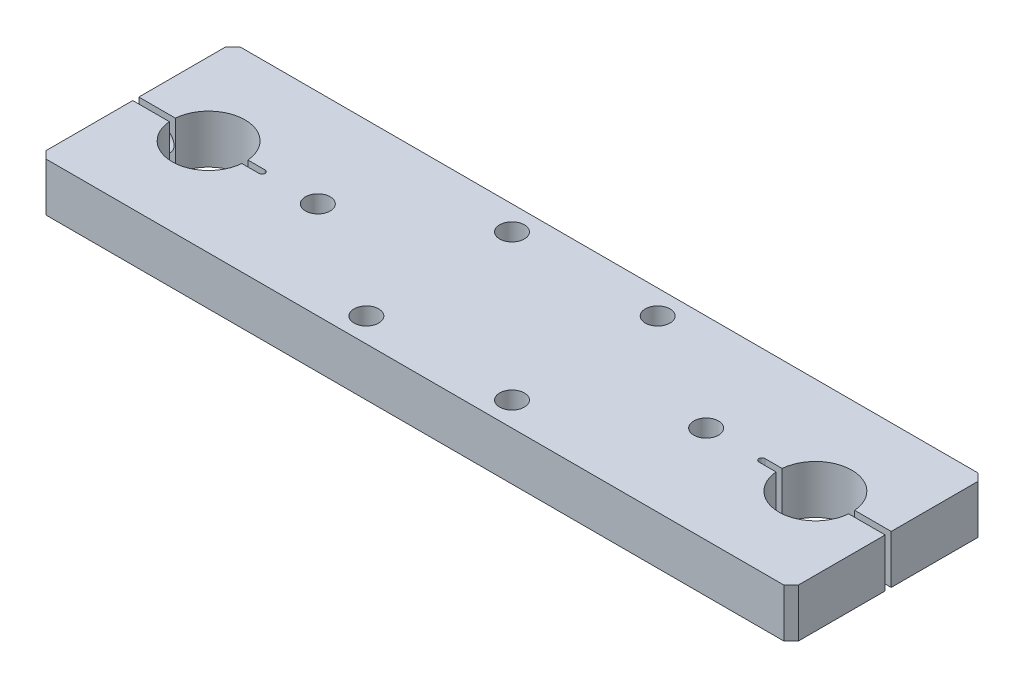
SolidWorks part; units mm, degrees
material "45#"
ref_plane "前基準面" through (0, 0, 0) normal (0, 0, 1) x (1, 0, 0)
ref_plane "上基準面" through (0, 0, 0) normal (0, 1, 0) x (1, 0, 0)
ref_plane "右基準面" through (0, 0, 0) normal (1, 0, 0) x (0, 0, -1)
sketch "草图1" plane through (0, 0, 0) normal (0, 1, 0) x (1, 0, 0)
  line L1 (-155, -40) -> (155, -40)
  line L2 (-155, -40) -> (-155, 40)
  line L3 (-155, 40) -> (155, 40)
  line L4 (155, -40) -> (155, 40)
  line L5 (-155, -40) -> (155, 40) construction
  line L6 (-155, 40) -> (155, -40) construction
  point P0 (0, 0)
  dimension "D1" = 310
  dimension "D2" = 80
extrude "凸台-拉伸1" add sketch "草图1" along normal mid plane 20
sketch "草图2" plane through (0, 10, 0) normal (0, 1, 0) x (1, 0, 0)
  line L0 (0, -60.9289) -> (0, 0) construction
  circle A0 centre (125, 0) radius 15
  circle A1 centre (-125, 0) radius 15
  dimension "D1" = 30
  dimension "D2" = 250
extrude "切除-拉伸1" cut sketch "草图2" against normal up to surface (20 mm away) up to face at (0, -10, 0)
chamfer "倒角1" distance 3 angle 45 4 edges at (-155, 0, 40) (-155, 0, -40) (155, 0, 40) (155, 0, -40)
sketch "草图3" plane through (0, 10, 0) normal (0, 1, 0) x (1, 0, 0)
  line L0 (155, 0) -> (103, 0) construction
  line L1 (155, -37) -> (155, 37) construction
  line L2 (155, -1.25) -> (103, -1.25)
  line L3 (155, 1.25) -> (103, 1.25)
  line L4 (0, -106.744) -> (0, 0) construction
  line L5 (-155, 0) -> (-103, 0) construction
  line L6 (-155, -1.25) -> (-103, -1.25)
  line L7 (-155, 1.25) -> (-103, 1.25)
  arc A0 (155, -1.25) -> (155, 1.25) centre (155, 0) ccw
  arc A1 (103, 1.25) -> (103, -1.25) centre (103, 0) ccw
  arc A2 (-155, -1.25) -> (-155, 1.25) centre (-155, 0) cw
  arc A3 (-103, 1.25) -> (-103, -1.25) centre (-103, 0) cw
  circle A4 centre (125, 0) radius 15 construction
  point P5 (129, 0)
  point P14 (-129, 0)
  dimension "D2" = 22
  dimension "D1" = 2.5
extrude "切除-拉伸2" cut sketch "草图3" against normal up to surface (20 mm away) up to face at (125, -10, -15)
hole_wizard "打孔尺寸(%根据)内六角圆柱头螺钉的类型2" positions "草图4" profile "草图5" counterbore size "M8" standard "GB"
sketch "草图4" plane through (0, 0, -40) normal (0, 0, -1) x (-1, 0, 0)
  line L0 (0, 76.1314) -> (0, 0) construction
  line L1 (-155, -10) -> (-155, 10) construction
  point P0 (-145, 0)
  point P6 (145, 0)
  dimension "D1" = 10
sketch "草图5" plane through (145, 0, -40) normal (1, 0, 0) x (0, 1, 0)
  line L0 (0, 0) -> (0, 42.7039)
  line L1 (0, 42.7039) -> (4.5, 40)
  line L2 (4.5, 40) -> (4.5, 9)
  line L3 (4.5, 9) -> (7.5, 9)
  line L4 (7.5, 9) -> (7.5, 0)
  line L5 (7.5, 0) -> (0, 0)
  line L10 (0, 42.7039) -> (-4.5, 40) construction
  line L11 (0, -6.35) -> (0, 107.95) construction
  dimension "孔直径" = 9
  dimension "孔深度" = 40
  dimension "柱形沉头孔直径" = 15
  dimension "柱形沉头孔深度" = 9
  dimension "导头角度" = 118
hole_wizard "M8 螺纹孔1" positions "草图6" profile "草图7" tap size "M8" standard "GB"
sketch "草图6" plane through (0, 0, 1.25) normal (0, 0, -1) x (-1, 0, 0)
  point P0 (-145, 0)
  point P4 (145, 0)
sketch "草图7" plane through (145, 0, 1.25) normal (1, 0, 0) x (0, 1, 0)
  line L0 (0, 0) -> (0, 21.7929)
  line L1 (0, 21.7929) -> (3.4, 19.75)
  line L2 (3.4, 19.75) -> (3.4, 0)
  line L5 (3.4, 0) -> (0, 0)
  line L10 (0, 21.7929) -> (-3.4, 19.75) construction
  line L11 (0, -6.35) -> (0, 107.95) construction
  dimension "螺纹孔钻头直径" = 6.8
  dimension "螺纹孔钻头深度" = 19.75
  dimension "导头角度" = 118
cosmetic thread "孔螺蚊线1" parameters "D1"=16, "D2"=8
cosmetic thread "孔螺蚊线2" parameters "D1"=16, "D2"=8
hole_wizard "打孔尺寸(%根据)内六角圆柱头螺钉的类型2" positions "草图8" profile "草图9" counterbore size "M10" standard "GB"
sketch "草图8" plane through (0, -10, 0) normal (0, -1, 0) x (-1, 0, 0)
  line L0 (0, 59.2354) -> (0, 0) construction
  line L1 (0, 0) -> (-105.2792, 0) construction
  point P0 (-30, 30)
  point P12 (30, 30)
  point P13 (30, -30)
  point P14 (-30, -30)
  dimension "D1" = 60
  dimension "D2" = 60
sketch "草图9" plane through (30, -10, -30) normal (1, 0, 0) x (0, 0, -1)
  line L0 (0, 0) -> (0, 23.0547)
  line L1 (0, 23.0547) -> (5.5, 19.75)
  line L2 (5.5, 19.75) -> (5.5, 11)
  line L3 (5.5, 11) -> (9, 11)
  line L4 (9, 11) -> (9, 0)
  line L5 (9, 0) -> (0, 0)
  line L10 (0, 23.0547) -> (-5.5, 19.75) construction
  line L11 (0, -6.35) -> (0, 107.95) construction
  dimension "孔直径" = 11
  dimension "孔深度" = 19.75
  dimension "柱形沉头孔直径" = 18
  dimension "柱形沉头孔深度" = 11
  dimension "导头角度" = 118
hole_wizard "M12 螺纹孔1" positions "草图10" profile "草图11" tap size "M12" standard "GB" end condition through all
sketch "草图10" plane through (0, 10, 0) normal (0, 1, 0) x (1, 0, 0)
  line L0 (0, -54.1617) -> (0, 0) construction
  point P0 (80, 0)
  point P8 (-80, 0)
  dimension "D1" = 160
sketch "草图11" plane through (80, 10, 0) normal (1, 0, 0) x (0, 0, 1)
  line L0 (0, 0) -> (0, 20)
  line L1 (0, 20) -> (5.1, 20)
  line L2 (5.1, 20) -> (5.1, 0)
  line L5 (5.1, 0) -> (0, 0)
  line L11 (0, -6.35) -> (0, 107.95) construction
  dimension "通孔螺纹孔钻头直径" = 10.2
  dimension "通孔螺纹孔钻头深度" = 20
cosmetic thread "孔螺蚊线3" parameters "D2"=12
cosmetic thread "孔螺蚊线4" parameters "D2"=12
